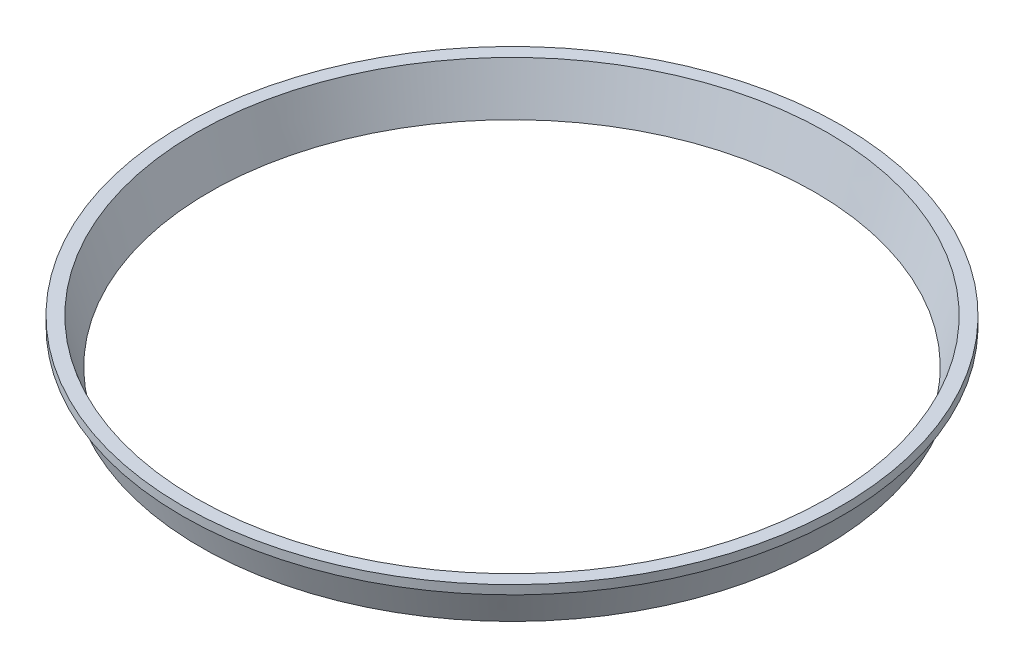
SolidWorks part; units mm, degrees
ref_plane "Front plane" through (0, 0, 0) normal (0, 0, 1) x (1, 0, 0)
ref_plane "Top plane" through (0, 0, 0) normal (0, 1, 0) x (1, 0, 0)
ref_plane "Right plane" through (0, 0, 0) normal (1, 0, 0) x (0, 0, -1)
sketch "Sketch 5" plane through (0, 0, 0) normal (0, 0, 1) x (1, 0, 0)
  line L0 (-74, 10) -> (-74, 8)
  line L1 (-74, 8) -> (-72.4, 8)
  line L2 (-72.4, 8) -> (-70, 0)
  line L3 (-70, 0) -> (-68, 0)
  line L4 (-68, 0) -> (-71, 10)
  line L5 (-71, 10) -> (-74, 10)
  line L6 (-68, 0) -> (0, 0)
  line L7 (0, 0) -> (0, 21.0982) construction
  dimension "D1" = 74
  dimension "D2" = 71
  dimension "D3" = 70
  dimension "D4" = 68
  dimension "D5" = 2
  dimension "D6" = 8
revolve "Revolve 1" add sketch "Sketch 5" angle 360 about L7
